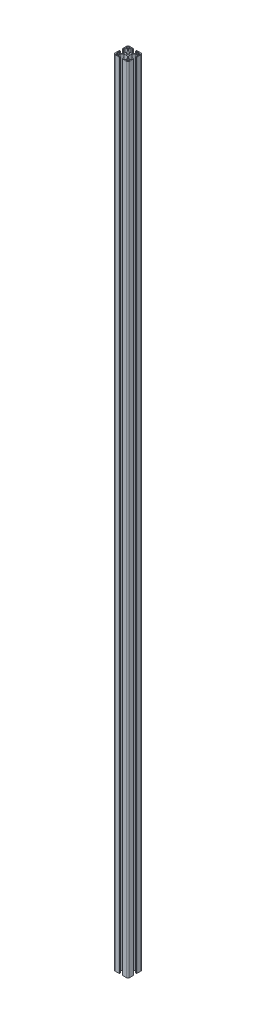
from build123d import *

# Parameters (mm, degrees)
SKETCH1_R                 = 3.4
F_40_X_40L_X_R4_5_1_DEPTH = 2200


with BuildPart() as part:
    # Sketch1 → 铝型材 40 X 40L X R4.5(1) (new body)
    with BuildSketch(Plane(origin=(0, 0, 0), x_dir=(-1, 0, 0), z_dir=(0, 1, 0))):
        with BuildLine():
            Line((-5.1, 20), (-5.1, 19.5))
            Line((-5.1, 19.5), (-4.1, 19.5))
            Line((-4.1, 19.5), (-4.1, 17))
            Line((-4.1, 17), (-6.1, 17))
            Line((-6.1, 17), (-6.1, 18.5))
            Line((-6.1, 18.5), (-10.3, 18.5))
            Line((-10.3, 18.5), (-10.3, 11.3))
            Line((-10.3, 11.3), (-5, 6))
            Line((-5, 6), (5, 6))
            Line((5, 6), (10.3, 11.3))
            Line((10.3, 11.3), (10.3, 18.5))
            Line((10.3, 18.5), (6.1, 18.5))
            Line((6.1, 18.5), (6.1, 17))
            Line((6.1, 17), (4.1, 17))
            Line((4.1, 17), (4.1, 19.5))
            Line((4.1, 19.5), (5.1, 19.5))
            Line((5.1, 19.5), (5.1, 20))
            Line((5.1, 20), (15.5, 20))
            ThreePointArc((15.5, 20), (18.681980515, 18.681980515), (20, 15.5))
            Line((20, 15.5), (20, 5.1))
            Line((20, 5.1), (19.5, 5.1))
            Line((19.5, 5.1), (19.5, 4.1))
            Line((19.5, 4.1), (17, 4.1))
            Line((17, 4.1), (17, 6.1))
            Line((17, 6.1), (18.5, 6.1))
            Line((18.5, 6.1), (18.5, 10.3))
            Line((18.5, 10.3), (11.3, 10.3))
            Line((11.3, 10.3), (6, 5))
            Line((6, 5), (6, -5))
            Line((6, -5), (11.3, -10.3))
            Line((11.3, -10.3), (18.5, -10.3))
            Line((18.5, -10.3), (18.5, -6.1))
            Line((18.5, -6.1), (17, -6.1))
            Line((17, -6.1), (17, -4.1))
            Line((17, -4.1), (19.5, -4.1))
            Line((19.5, -4.1), (19.5, -5.1))
            Line((19.5, -5.1), (20, -5.1))
            Line((20, -5.1), (20, -15.5))
            ThreePointArc((20, -15.5), (18.681980515, -18.681980515), (15.5, -20))
            Line((15.5, -20), (5.1, -20))
            Line((5.1, -20), (5.1, -19.5))
            Line((5.1, -19.5), (4.1, -19.5))
            Line((4.1, -19.5), (4.1, -17))
            Line((4.1, -17), (6.1, -17))
            Line((6.1, -17), (6.1, -18.5))
            Line((6.1, -18.5), (10.3, -18.5))
            Line((10.3, -18.5), (10.3, -11.3))
            Line((10.3, -11.3), (5, -6))
            Line((5, -6), (-5, -6))
            Line((-5, -6), (-10.3, -11.3))
            Line((-10.3, -11.3), (-10.3, -18.5))
            Line((-10.3, -18.5), (-6.1, -18.5))
            Line((-6.1, -18.5), (-6.1, -17))
            Line((-6.1, -17), (-4.1, -17))
            Line((-4.1, -17), (-4.1, -19.5))
            Line((-4.1, -19.5), (-5.1, -19.5))
            Line((-5.1, -19.5), (-5.1, -20))
            Line((-5.1, -20), (-15.5, -20))
            ThreePointArc((-15.5, -20), (-18.681980515, -18.681980515), (-20, -15.5))
            Line((-20, -15.5), (-20, -5.1))
            Line((-20, -5.1), (-19.5, -5.1))
            Line((-19.5, -5.1), (-19.5, -4.1))
            Line((-19.5, -4.1), (-17, -4.1))
            Line((-17, -4.1), (-17, -6.1))
            Line((-17, -6.1), (-18.5, -6.1))
            Line((-18.5, -6.1), (-18.5, -10.3))
            Line((-18.5, -10.3), (-11.3, -10.3))
            Line((-11.3, -10.3), (-6, -5))
            Line((-6, -5), (-6, 5))
            Line((-6, 5), (-11.3, 10.3))
            Line((-11.3, 10.3), (-18.5, 10.3))
            Line((-18.5, 10.3), (-18.5, 6.1))
            Line((-18.5, 6.1), (-17, 6.1))
            Line((-17, 6.1), (-17, 4.1))
            Line((-17, 4.1), (-19.5, 4.1))
            Line((-19.5, 4.1), (-19.5, 5.1))
            Line((-19.5, 5.1), (-20, 5.1))
            Line((-20, 5.1), (-20, 15.5))
            ThreePointArc((-20, 15.5), (-18.681980515, 18.681980515), (-15.5, 20))
            Line((-15.5, 20), (-5.1, 20))
        make_face()
        Circle(SKETCH1_R, mode=Mode.SUBTRACT)
        with BuildLine():
            Line((11.8, 17.5), (15, 17.5))
            ThreePointArc((15, 17.5), (16.767766953, 16.767766953), (17.5, 15))
            Line((17.5, 15), (17.5, 11.8))
            Line((17.5, 11.8), (11.8, 11.8))
            Line((11.8, 11.8), (11.8, 17.5))
        make_face(mode=Mode.SUBTRACT)
        with BuildLine():
            Line((-15, 17.5), (-11.8, 17.5))
            Line((-11.8, 17.5), (-11.8, 11.8))
            Line((-11.8, 11.8), (-17.5, 11.8))
            Line((-17.5, 11.8), (-17.5, 15))
            ThreePointArc((-17.5, 15), (-16.767766953, 16.767766953), (-15, 17.5))
        make_face(mode=Mode.SUBTRACT)
        with BuildLine():
            Line((-17.5, -11.8), (-11.8, -11.8))
            Line((-11.8, -11.8), (-11.8, -17.5))
            Line((-11.8, -17.5), (-15, -17.5))
            ThreePointArc((-15, -17.5), (-16.767766953, -16.767766953), (-17.5, -15))
            Line((-17.5, -15), (-17.5, -11.8))
        make_face(mode=Mode.SUBTRACT)
        with BuildLine():
            Line((11.8, -11.8), (17.5, -11.8))
            Line((17.5, -11.8), (17.5, -15))
            ThreePointArc((17.5, -15), (16.767766953, -16.767766953), (15, -17.5))
            Line((15, -17.5), (11.8, -17.5))
            Line((11.8, -17.5), (11.8, -11.8))
        make_face(mode=Mode.SUBTRACT)
    extrude(amount=F_40_X_40L_X_R4_5_1_DEPTH)


solid = part.part
